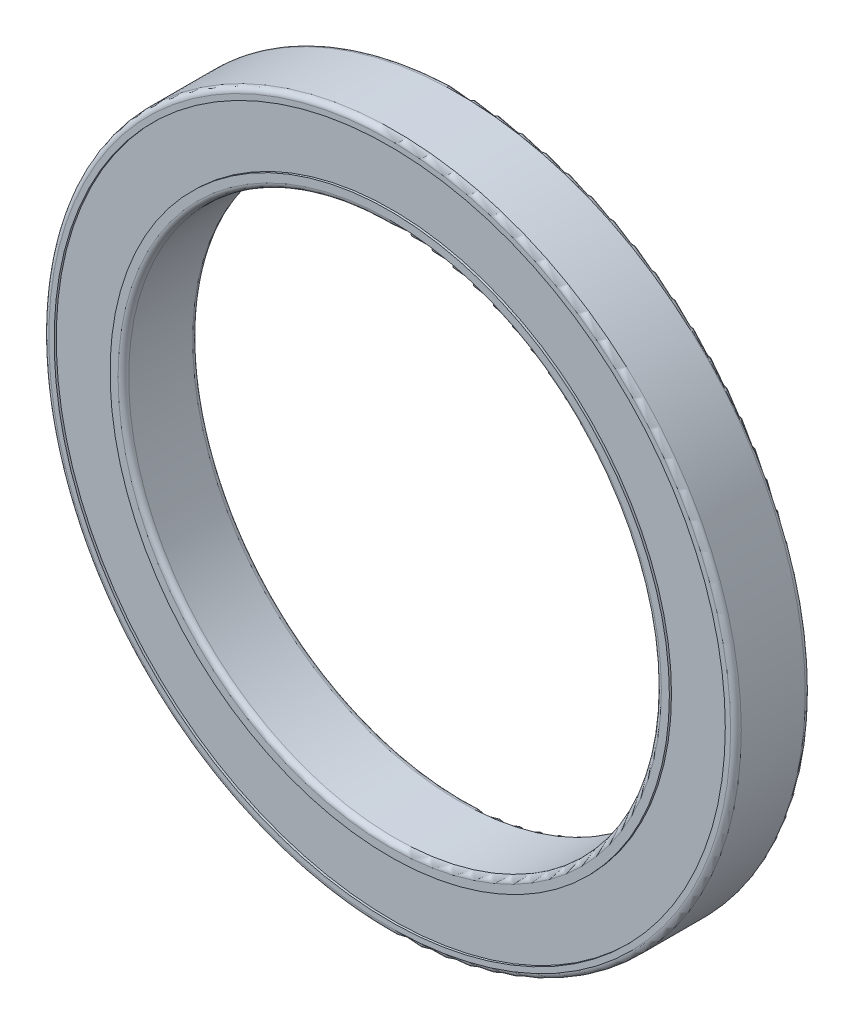
SolidWorks part; units mm, degrees
material "AISI 304"
ref_plane "Front Plane" through (0, 0, 0) normal (0, 0, 1) x (1, 0, 0)
ref_plane "Top Plane" through (0, 0, 0) normal (0, 1, 0) x (1, 0, 0)
ref_plane "Right Plane" through (0, 0, 0) normal (1, 0, 0) x (0, 0, -1)
sketch "Sketch1" plane through (0, 0, 0) normal (0, 0, 1) x (1, 0, 0)
  circle A0 centre (0, 0) radius 25
  circle A1 centre (0, 0) radius 32.5
  dimension "D1" = 50
  dimension "D2" = 65
extrude "Boss-Extrude1" add sketch "Sketch1" along normal mid plane 7
sketch "Sketch2" plane through (0, 0, 3.5) normal (0, 0, 1) x (1, 0, 0)
  circle A0 centre (0, 0) radius 26.25
  circle A1 centre (0, 0) radius 31.5
  dimension "D1" = 52.5
  dimension "D2" = 63
extrude "Cut-Extrude1" cut sketch "Sketch2" against normal blind 0.2
mirror "Mirror1" about plane through (0, 0, 0) normal (0, 0, 1) of "Cut-Extrude1"
fillet "Fillet1" radius 0.5 4 edges at (32.5, 0, -3.5) (32.5, 0, 3.5) (25, 0, -3.5) (25, 0, 3.5)
